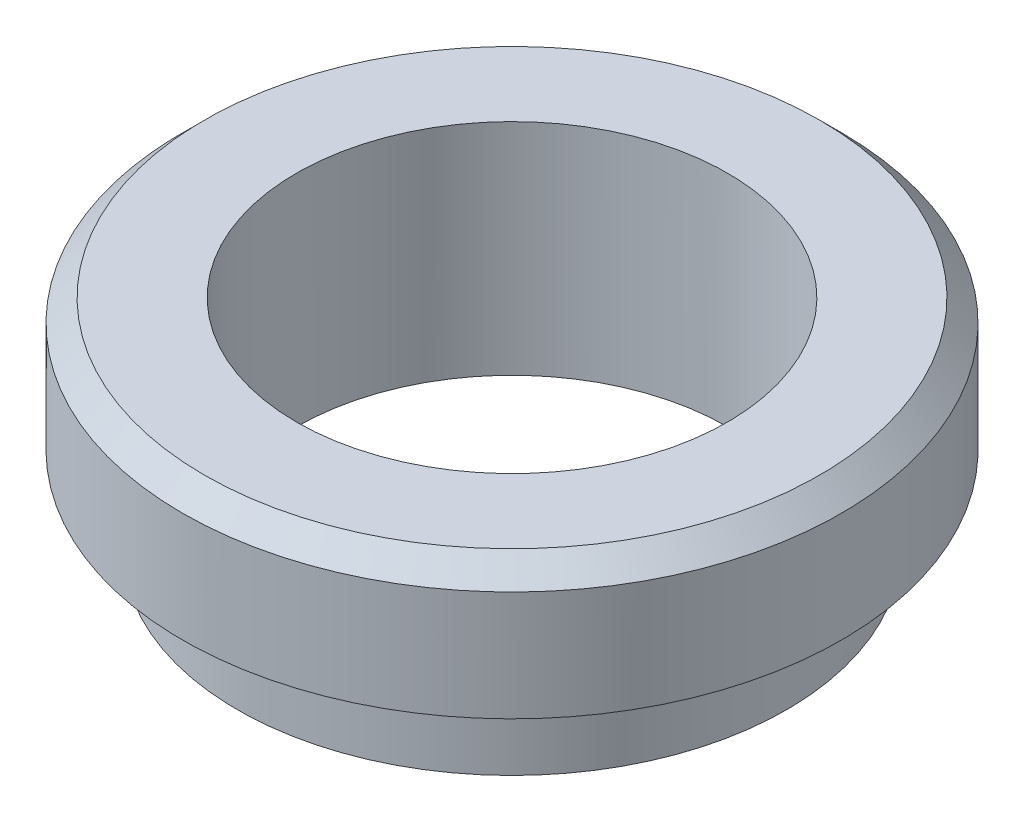
from build123d import *

# Parameters (mm, degrees)
G1_1_4_TAPPED_HOLE1_D     = 39.25
G1_1_4_TAPPED_HOLE1_DEPTH = 90.75
G1_1_4_TAPPED_HOLE1_TIP   = 11.791889648
CHAMFER1_SIZE             = 2


with BuildPart() as part:
    # Sketch1 → Revolve1 (revolve)
    with BuildSketch(Plane.XY, mode=Mode.PRIVATE) as revolve1_sk:
        Polygon((0, 0), (30, 0), (30, -12), (25, -12), (25, -20), (0, -20), align=None)
    revolve(revolve1_sk.sketch.rotate(Axis((0, -20, 0), (0, 1, 0)), 90), axis=Axis((0, -20, 0), (0, 1, 0)))

    # G1-1/4 Tapped Hole1
    with Locations(Plane(origin=(0, 0, 0), x_dir=(1, 0, 0), z_dir=(0, 1, 0))):
        with Locations((0, 0)):
            Hole(G1_1_4_TAPPED_HOLE1_D / 2, depth=G1_1_4_TAPPED_HOLE1_DEPTH)
            with Locations((0, 0, -(G1_1_4_TAPPED_HOLE1_DEPTH + G1_1_4_TAPPED_HOLE1_TIP / 2))):  # 118° drill point
                Cone(0, G1_1_4_TAPPED_HOLE1_D / 2, G1_1_4_TAPPED_HOLE1_TIP, mode=Mode.SUBTRACT)

    # Chamfer1
    chamfer1_edges = [part.edges().sort_by_distance(p)[0] for p in [
        (0, 0, 30),
    ]]
    chamfer(chamfer1_edges, length=CHAMFER1_SIZE)


solid = part.part
